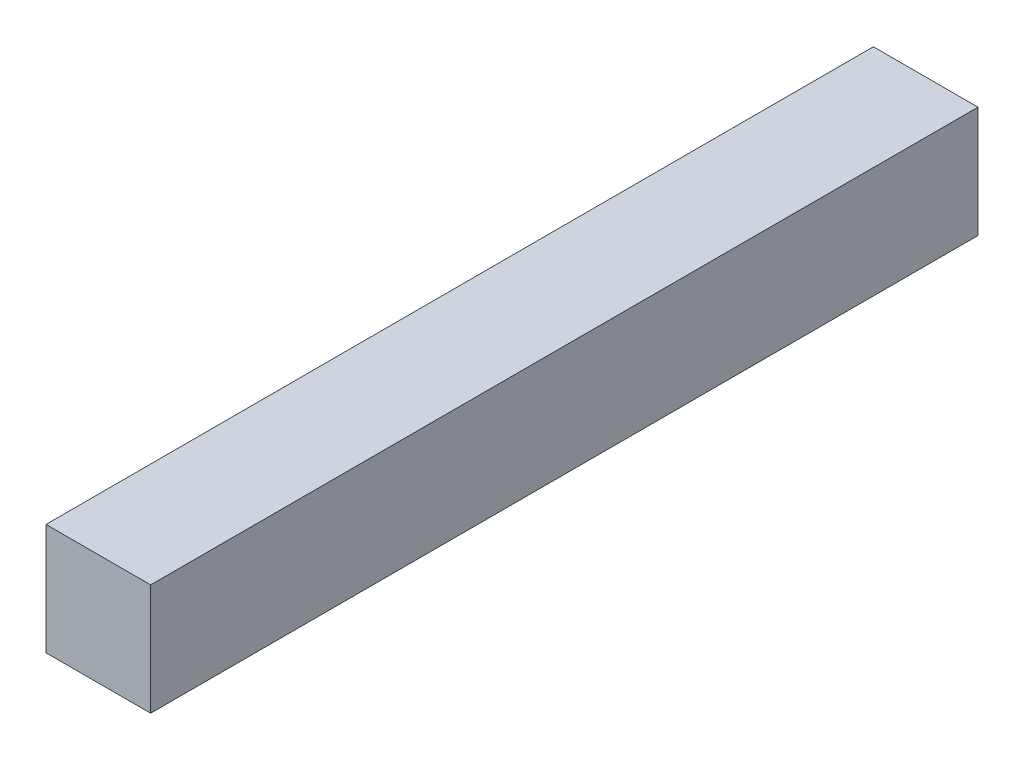
SolidWorks part; units mm, degrees
ref_plane "前视基准面" through (0, 0, 0) normal (0, 0, 1) x (1, 0, 0)
ref_plane "上视基准面" through (0, 0, 0) normal (0, 1, 0) x (1, 0, 0)
ref_plane "右视基准面" through (0, 0, 0) normal (1, 0, 0) x (0, 0, -1)
sketch "草图1" plane through (0, 0, 0) normal (0, 0, 1) x (1, 0, 0)
  line L1 (-16, -17) -> (16, -17)
  line L2 (-16, -17) -> (-16, 17)
  line L3 (-16, 17) -> (16, 17)
  line L4 (16, -17) -> (16, 17)
  line L5 (-16, -17) -> (16, 17) construction
  line L6 (-16, 17) -> (16, -17) construction
  point P0 (0, 0)
  dimension "D1" = 32
  dimension "D2" = 34
extrude "凸台-拉伸1" add sketch "草图1" along normal blind 253
